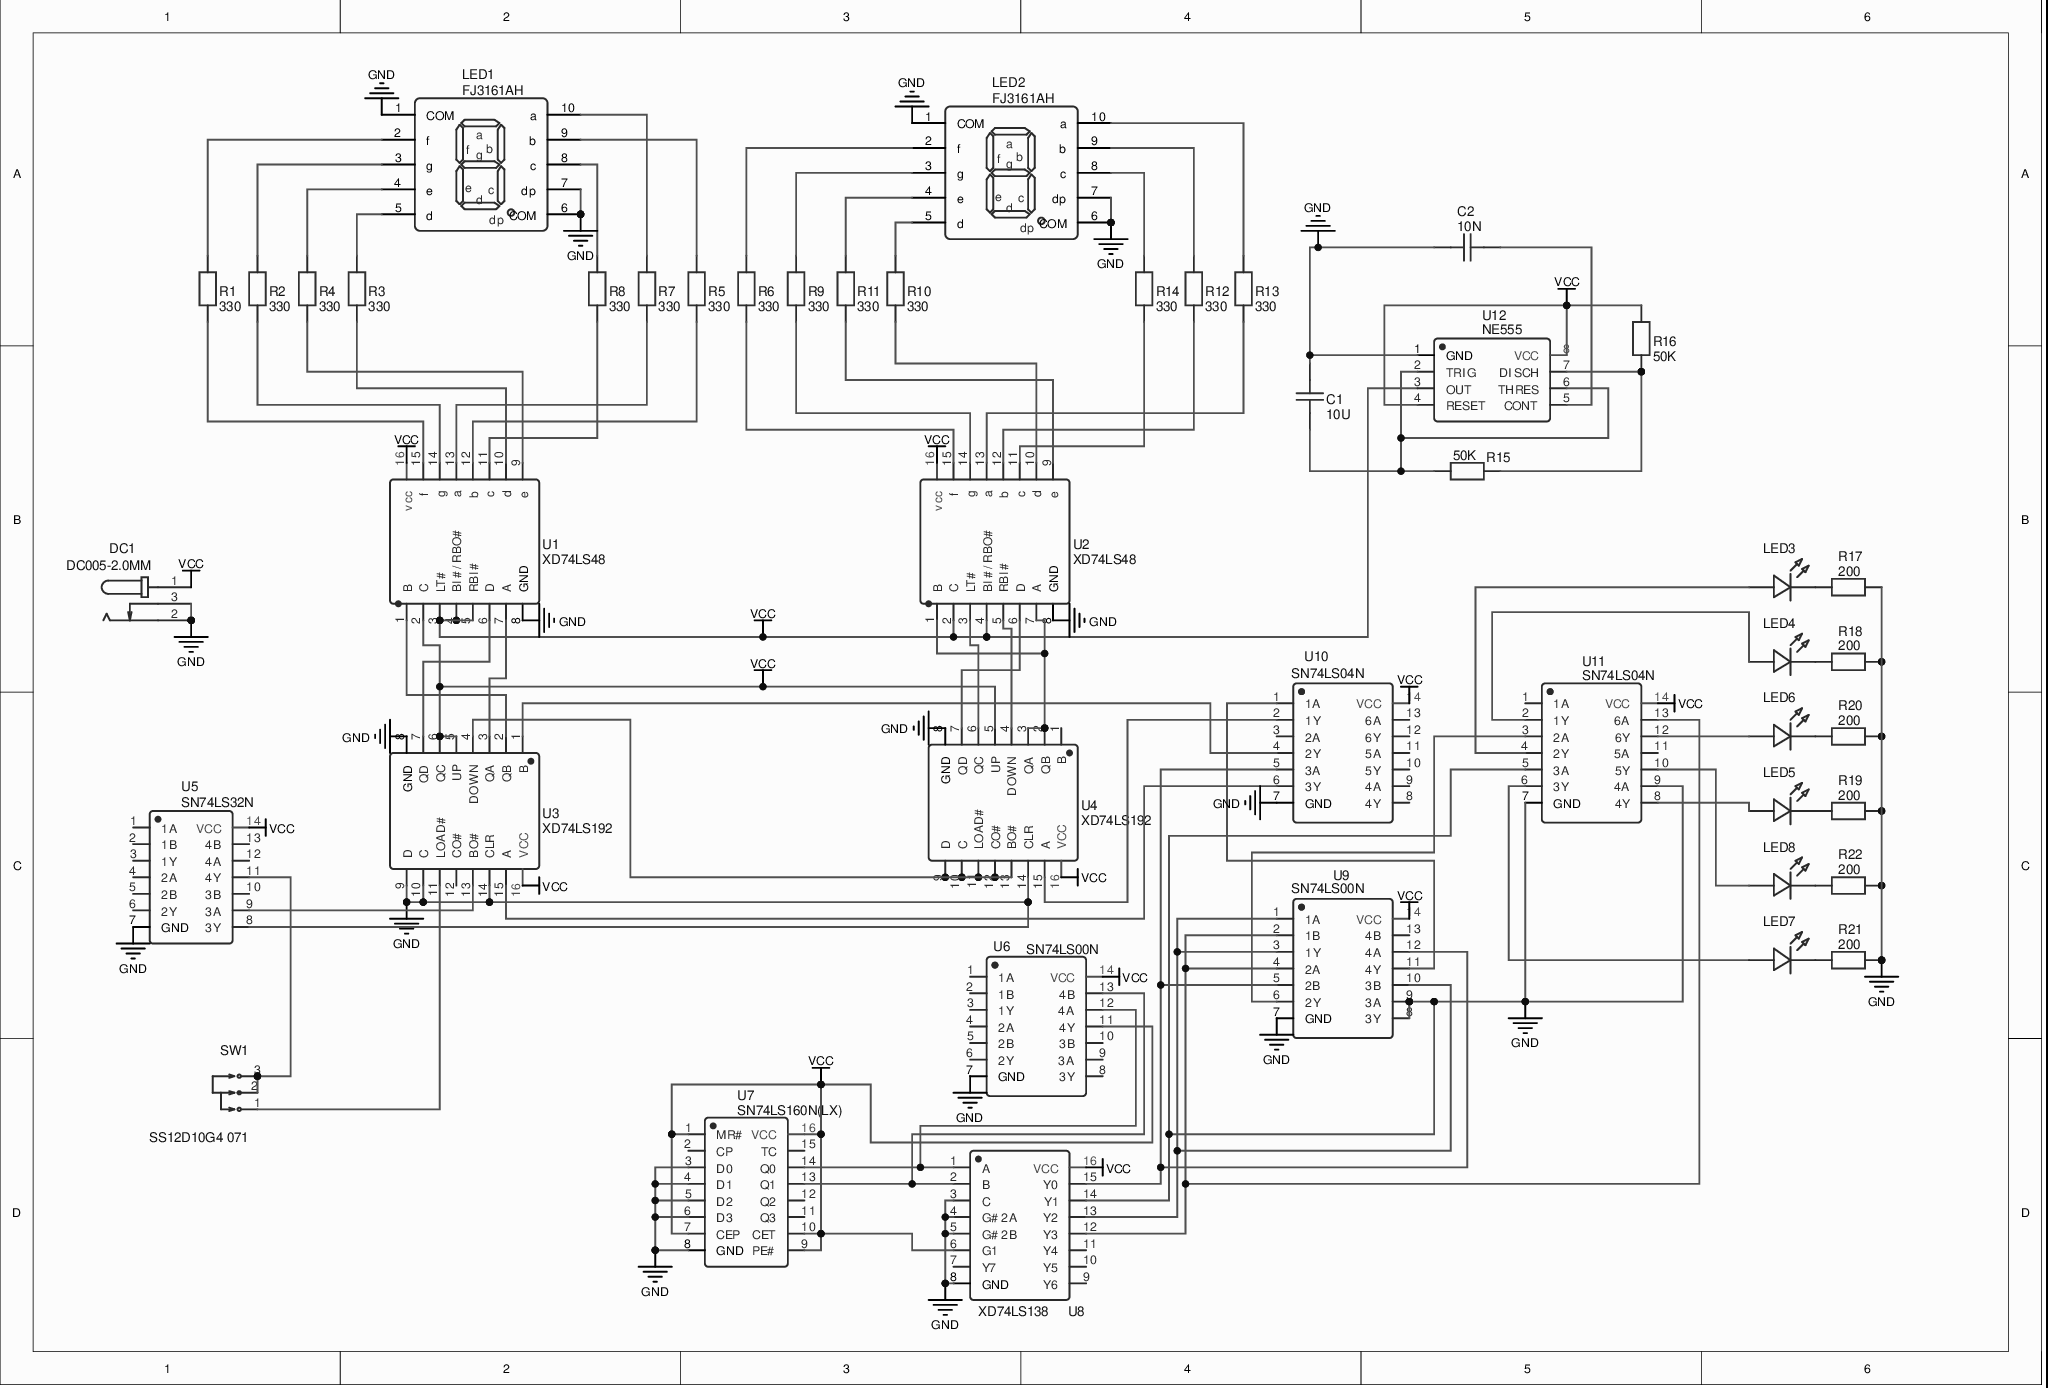
[diagram p0: MISC80800-4.schdoc]
# Altium project MISC80800-7.PrjPcb
1 sheet, 46 parts. Net scope: global (net labels, ports and power ports of the same name join across sheets).
Board file: MISC80800.pcbdoc

## Sheet MISC80800-4.schdoc
size 312 x 212 mm

### Parts
C1  10U  [RAD-0.2]
C2  10N  [RAD-0.2]
DC1  DC005-2.0MM  [DC-IN-TH_DC005]
LED1  FJ3161AH  [LED-SEG-TH_10P-L14.0-W7.5-P2.54-S5.08-TL]
LED2  FJ3161AH  [LED-SEG-TH_10P-L14.0-W7.5-P2.54-S5.08-TL]
LED3  LED-TH-5mm_R  [LED-TH_BD5.0_RED]  (value not drawn)
LED4  LED-TH-5mm_R  [LED-TH_BD5.0_RED]  (value not drawn)
LED5  LED-TH-5mm_R  [LED-TH_BD5.0_RED]  (value not drawn)
LED6  LED-TH-5mm_R  [LED-TH_BD5.0_RED]  (value not drawn)
LED7  LED-TH-5mm_R  [LED-TH_BD5.0_RED]  (value not drawn)
LED8  LED-TH-5mm_R  [LED-TH_BD5.0_RED]  (value not drawn)
R1  330  [R_AXIAL-0.4]
R2  330  [R_AXIAL-0.4]
R3  330  [R_AXIAL-0.4]
R4  330  [R_AXIAL-0.4]
R5  330  [R_AXIAL-0.4]
R6  330  [R_AXIAL-0.4]
R7  330  [R_AXIAL-0.4]
R8  330  [R_AXIAL-0.4]
R9  330  [R_AXIAL-0.4]
R10  330  [R_AXIAL-0.4]
R11  330  [R_AXIAL-0.4]
R12  330  [R_AXIAL-0.4]
R13  330  [R_AXIAL-0.4]
R14  330  [R_AXIAL-0.4]
R15  50K  [R_AXIAL-0.4]
R16  50K  [R_AXIAL-0.4]
R17  200  [R_AXIAL-0.4]
R18  200  [R_AXIAL-0.4]
R19  200  [R_AXIAL-0.4]
R20  200  [R_AXIAL-0.4]
R21  200  [R_AXIAL-0.4]
R22  200  [R_AXIAL-0.4]
SW1  SS12D10G4 071  [SW-TH_SHOU-HAN_SS12D10G4]
U1  XD74LS48  [DIP-16_L19.3-W6.4-P2.54-LS7.6-BL]
U2  XD74LS48  [DIP-16_L19.3-W6.4-P2.54-LS7.6-BL]
U3  XD74LS192  [DIP-16_L19.3-W6.4-P2.54-LS7.6-BL]
U4  XD74LS192  [DIP-16_L19.3-W6.4-P2.54-LS7.6-BL]
U5  SN74LS32N  [PDIP-14_L19.6-W6.5-P2.54-LS7.9-BL]
U6  SN74LS00N  [PDIP-14_L19.7-W6.6-P2.54-LS8.3-BL]
U7  SN74LS160N(LX)  [DIP-16_L22.4-W6.4-P2.54-LS8.64-BL]
U8  XD74LS138  [DIP-16_L19.8-W6.5-P2.54-LS7.6-BL]
U9  SN74LS00N  [PDIP-14_L19.7-W6.6-P2.54-LS8.3-BL]
U10  SN74LS04N  [PDIP-14_L19.7-W6.6-P2.54-LS8.3-BL]
U11  SN74LS04N  [PDIP-14_L19.7-W6.6-P2.54-LS8.3-BL]
U12  NE555  [DIP-8_L9.8-W6.6-P2.54-LS7.6-BL]

### Nets
GND: C1.2 C2.2 DC1.2 DC1.3 LED1.1(COM) LED1.6(COM) LED1.7(dp) LED2.1(COM) LED2.6(COM) LED2.7(dp) R17.2 R18.2 R19.2 R20.2 R21.2 R22.2 U1.8(GND) U2.8(GND) U3.8(GND) U3.9(D) U3.10(C) U3.14(CLR) U4.8(GND) U4.14(CLR) U5.7(GND) U5.8(3Y) U6.7(GND) U7.3(D0) U7.4(D1) U7.5(D2) U7.6(D3) U7.8(GND) U8.3(C) U8.4(G#2A) U8.5(G#2B) U8.8(GND) U8.14(Y1) U9.7(GND) U9.8(3Y) U9.9(3A) U10.7(GND) U11.5(3A) U11.7(GND) U11.9(4A) U12.1(GND)
VCC: DC1.1 R16.1 U1.2(C) U1.3(LT#) U1.4(BI#/RBO#) U1.5(RBI#) U1.16(vcc) U2.2(C) U2.4(BI#/RBO#) U2.16(vcc) U3.5(UP) U3.6(QC) U3.16(VCC) U4.5(UP) U4.16(VCC) U5.14(VCC) U6.11(4Y) U6.14(VCC) U7.1(MR#) U7.7(CEP) U7.9(PE#) U7.10(CET) U7.16(VCC) U8.6(G1) U8.16(VCC) U9.14(VCC) U10.14(VCC) U11.14(VCC) U12.3(OUT) U12.4(RESET) U12.8(VCC)
NetC1_1: C1.1 R15.2 U12.2(TRIG) U12.6(THRES)
NetC2_1: C2.1 U12.5(CONT)
NetLED1_2: LED1.2(f) R1.2
NetLED1_3: LED1.3(g) R2.2
NetLED1_4: LED1.4(e) R4.2
NetLED1_5: LED1.5(d) R3.2
NetLED1_8: LED1.8(c) R8.2
NetLED1_9: LED1.9(b) R5.2
NetLED1_10: LED1.10(a) R7.2
NetLED2_2: LED2.2(f) R6.2
NetLED2_3: LED2.3(g) R9.2
NetLED2_4: LED2.4(e) R11.2
NetLED2_5: LED2.5(d) R10.2
NetLED2_8: LED2.8(c) R14.2
NetLED2_9: LED2.9(b) R12.2
NetLED2_10: LED2.10(a) R13.2
NetLED3_1: LED3.1 U11.4(2Y)
NetLED3_2: LED3.2 R17.1
NetLED4_1: LED4.1 U11.2(1Y)
NetLED4_2: LED4.2 R18.1
NetLED5_1: LED5.1 U11.8(4Y)
NetLED5_2: LED5.2 R19.1
NetLED6_1: LED6.1 U11.12(6Y)
NetLED6_2: LED6.2 R20.1
NetLED7_1: LED7.1 U11.6(3Y)
NetLED7_2: LED7.2 R21.1
NetLED8_1: LED8.1 U11.10(5Y)
NetLED8_2: LED8.2 R22.1
NetR1_1: R1.1 U1.15(f)
NetR2_1: R2.1 U1.14(g)
NetR3_1: R3.1 U1.10(d)
NetR4_1: R4.1 U1.9(e)
NetR5_1: R5.1 U1.12(b)
NetR6_1: R6.1 U2.15(f)
NetR7_1: R7.1 U1.13(a)
NetR8_1: R8.1 U1.11(c)
NetR9_1: R9.1 U2.14(g)
NetR10_1: R10.1 U2.10(d)
NetR11_1: R11.1 U2.9(e)
NetR12_1: R12.1 U2.12(b)
NetR13_1: R13.1 U2.13(a)
NetR14_1: R14.1 U2.11(c)
NetR15_1: R15.1 R16.2 U12.7(DISCH)
NetSW1_1: SW1.1 U3.11(LOAD#)
NetSW1_2: SW1.2 SW1.3 U5.11(4Y)
NetU1_1: U1.1(B) U3.2(QB)
NetU1_6: U1.6(D) U3.7(QD)
NetU1_7: U1.7(A) U3.3(QA)
NetU2_1: U2.1(B) U2.7(A) U4.2(QB) U4.3(QA)
NetU2_3: U2.3(LT#) U4.6(QC)
NetU2_5: U2.5(RBI#) U4.4(DOWN)
NetU2_6: U2.6(D) U4.7(QD)
NetU3_1: U3.1(B) U10.4(2Y)
NetU3_4: U3.4(DOWN) U4.9(D) U4.10(C) U4.11(LOAD#) U4.12(CO#) U4.13(BO#)
NetU3_13: U3.13(BO#) U5.9(3A)
NetU3_15: U3.15(A) U10.6(3Y)
NetU4_15: U4.15(A) U10.2(1Y)
NetU6_12: U6.12(4A) U7.14(Q0) U8.1(A)
NetU6_13: U6.13(4B) U7.13(Q1) U8.2(B)
NetU8_12: U8.12(Y3) U9.2(1B) U9.4(2A) U11.13(6A)
NetU8_13: U8.13(Y2) U9.1(1A) U9.3(1Y) U9.10(3B)
NetU8_15: U8.15(Y0) U9.5(2B) U9.12(4A) U10.5(3A)
NetU9_6: U9.6(2Y) U11.3(2A)
NetU9_11: U9.11(4Y) U10.1(1A)

Not connected (* = marked no-connect by the designer): U3 12(CO#)*; U4 1(B); U5 1(1A)* 2(1B)* 3(1Y)* 4(2A)* 5(2B)* 6(2Y)* 10(3B)* 12(4A)* 13(4B)*; U6 1(1A)* 2(1B)* 3(1Y)* 4(2A)* 5(2B)* 6(2Y)* 8(3Y)* 9(3A)* 10(3B)*; U7 2(CP)* 11(Q3)* 12(Q2)* 15(TC)*; U8 7(Y7)* 9(Y6)* 10(Y5)* 11(Y4)*; U9 13(4B); U10 3(2A) 8(4Y)* 9(4A)* 10(5Y)* 11(5A)* 12(6Y)* 13(6A)*; U11 1(1A) 11(5A)

### Library data of the parts
C1 = 10U: nameAlias: Value(F); Contributor: LCEDA_Lib; spicePre: C; spiceSymbolName: C_RAD-0.2_US
C2 = 10N: nameAlias: Value(F); Contributor: LCEDA_Lib; spicePre: C; spiceSymbolName: C_RAD-0.2_US
DC1 = DC005-2.0MM: Manufacturer: SOFNG; Supplier: LCSC; Manufacturer Part: DC005-2.0MM; Supplier Part: C111567; spicePre: D; spiceSymbolName: DC005-2.0MM
LED1 LED2 = FJ3161AH: Manufacturer: 志浩; Supplier: LCSC; Manufacturer Part: FJ3161AH; Supplier Part: C10684; JLCPCB Part Class: Extended Part; spicePre: L; spiceSymbolName: FJ3161AH
LED3-LED8 = LED-TH-5mm_R: Manufacturer: EVERLIGHT(台湾亿光); Manufacturer Part: 333-2SURD/S530-A3; Contributor: LCEDA_Lib; Supplier Part: C87271; Supplier: LCSC; spicePre: L; spiceSymbolName: LED-TH-5mm_R
R1-R14 = 330: nameAlias: Value(Ω); Contributor: LCEDA_Lib; spicePre: R; spiceSymbolName: R_AXIAL-0.4_EU
R15 R16 = 50K: nameAlias: Value(Ω); Contributor: LCEDA_Lib; spicePre: R; spiceSymbolName: R_AXIAL-0.4_EU
R17-R22 = 200: nameAlias: Value(Ω); Contributor: LCEDA_Lib; spicePre: R; spiceSymbolName: R_AXIAL-0.4_EU
SW1 = SS12D10G4 071: Manufacturer: SHOU HAN(首韩); Contributor: LCSC; Supplier: LCSC; Supplier Part: C2887259; Manufacturer Part: SS12D10G4 071; JLCPCB Part Class: Extended Part; spicePre: S; spiceSymbolName: SS12D10G4 071
U1 U2 = XD74LS48: Manufacturer: XINLUDA(信路达); Contributor: LCSC; Supplier: LCSC; Supplier Part: C609759; Manufacturer Part: XD74LS48; JLCPCB Part Class: Extended Part; spicePre: U; spiceSymbolName: XD74LS48
U3 U4 = XD74LS192: Manufacturer: XINLUDA(信路达); Contributor: LCSC; Supplier: LCSC; Supplier Part: C609768; Manufacturer Part: XD74LS192; JLCPCB Part Class: Extended Part; spicePre: U; spiceSymbolName: XD74LS192
U5 = SN74LS32N: Manufacturer: TI(德州仪器); Contributor: LCSC; Supplier: LCSC; Supplier Part: C273644; Manufacturer Part: SN74LS32N; JLCPCB Part Class: Extended Part; spicePre: U; spiceSymbolName: SN74LS32N
U6 U9 = SN74LS00N: Manufacturer: TI(德州仪器); Contributor: LCSC; Supplier: LCSC; Manufacturer Part: SN74LS00N; Supplier Part: C181629; JLCPCB Part Class: Extended Part; spicePre: U; spiceSymbolName: SN74LS00N
U7 = SN74LS160N(LX): Manufacturer: LX(灵星芯微); Contributor: lcsc; Supplier: LCSC; Supplier Part: C22449620; Manufacturer Part: SN74LS160N(LX); JLCPCB Part Class: Extended Part; spicePre: U; spiceSymbolName: SN74LS160N(LX)
U8 = XD74LS138: Manufacturer: XINLUDA(信路达); Contributor: LCSC; Supplier: LCSC; Supplier Part: C513527; Manufacturer Part: XD74LS138; JLCPCB Part Class: Extended Part; spicePre: U; spiceSymbolName: XD74LS138
U10 U11 = SN74LS04N: Manufacturer: TI(德州仪器); Contributor: LCSC; Supplier: LCSC; Supplier Part: C183657; Manufacturer Part: SN74LS04N; JLCPCB Part Class: Extended Part; spicePre: U; spiceSymbolName: SN74LS04N
U12 = NE555: Manufacturer: TI(德州仪器); Manufacturer Part: NE555P; nameAlias: Value; Supplier: LCSC; Supplier Part: C46749; JLCPCB Part Class: Extended Part; spicePre: U; spiceSymbolName: NE555P